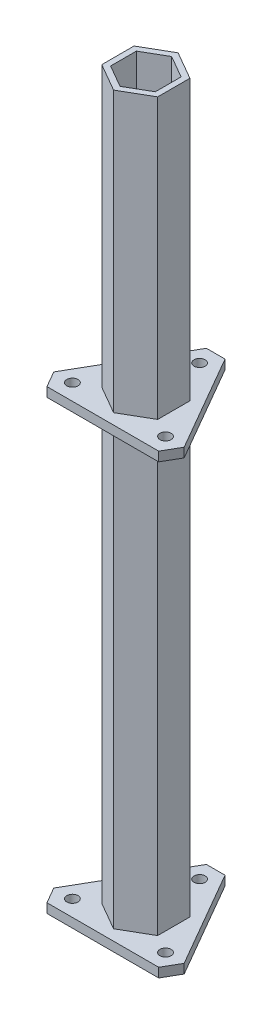
from build123d import *

# Parameters (mm, degrees)
BOSS_EXTRUDE1_DEPTH = 200
BOSS_EXTRUDE2_DEPTH = 5
CUT_EXTRUDE1_DEPTH  = 5
LPATTERN1_COUNT     = 4
LPATTERN1_PITCH     = 120
SKETCH5_R           = 3
CUT_EXTRUDE2_DEPTH  = 399.319386088
CUT_EXTRUDE4_DEPTH  = 10
CUT_EXTRUDE5_DEPTH  = 10


with BuildPart() as part:
    # Sketch1 → Boss-Extrude1 (new, symmetric)
    with BuildSketch(Plane(origin=(0, 0, 0), x_dir=(1, 0, 0), z_dir=(0, 1, 0))):
        Polygon((0, 17.320508076), (-15, 8.660254038), (-15, -8.660254038), (0, -17.320508076), (15, -8.660254038), (15, 8.660254038), align=None)
        Polygon((-12, 6.92820323), (-12, -6.92820323), (0, -13.856406461), (12, -6.92820323), (12, 6.92820323), (0, 13.856406461), align=None, mode=Mode.SUBTRACT)
    extrude(amount=BOSS_EXTRUDE1_DEPTH, both=True)

    # Sketch2 → Boss-Extrude2 (add)
    with BuildSketch(Plane(origin=(0, 170, 0), x_dir=(1, 0, 0), z_dir=(0, 1, 0))):
        Polygon((0, 46.188021535), (-40, -23.094010768), (40, -23.094010768), align=None)
        Polygon((15, 8.660254038), (0, 17.320508076), (-15, 8.660254038), (-15, -8.660254038), (0, -17.320508076), (15, -8.660254038), align=None, mode=Mode.SUBTRACT)
    boss_extrude2 = extrude(amount=-BOSS_EXTRUDE2_DEPTH)

    # Sketch3 → Cut-Extrude1 (cut)
    with BuildSketch(Plane.XZ.offset(-165)):
        Polygon((0, -46.188021535), (5, -37.527767497), (-5, -37.527767497), align=None)
        Polygon((40, 23.094010768), (30, 23.094010768), (35, 14.43375673), align=None)
        Polygon((-40, 23.094010768), (-35, 14.43375673), (-30, 23.094010768), align=None)
    cut_extrude1 = extrude(amount=-CUT_EXTRUDE1_DEPTH, mode=Mode.SUBTRACT)

    # LPattern1: Boss-Extrude2, Cut-Extrude1 ×4
    with Locations(*[(0, -i * LPATTERN1_PITCH, 0) for i in range(1, LPATTERN1_COUNT)]):
        add(boss_extrude2)
        add(cut_extrude1, mode=Mode.SUBTRACT)

    # Sketch5 → Cut-Extrude2 (cut, through all)
    with BuildSketch(Plane.XZ.offset(195)):
        with Locations(Location((-25, 14.43375673, 0), (0, 0, 270))):
            Circle(SKETCH5_R)
        with Locations(Location((25, 14.43375673, 0), (0, 0, 270))):
            Circle(SKETCH5_R)
        with Locations(Location((0, -28.867513459, 0), (0, 0, 270))):
            Circle(SKETCH5_R)
    extrude(amount=-CUT_EXTRUDE2_DEPTH, mode=Mode.SUBTRACT)

    # Sketch7 → Cut-Extrude4 (cut)
    with BuildSketch(Plane.XZ.offset(-165)):
        Polygon((30, 23.094010768), (-30, 23.094010768), (-35, 14.43375673), (-5, -37.527767497), (5, -37.527767497), (35, 14.43375673), align=None)
        Polygon((-15, -8.660254038), (-15, 8.660254038), (0, 17.320508076), (15, 8.660254038), (15, -8.660254038), (0, -17.320508076), align=None, mode=Mode.SUBTRACT)
    extrude(amount=-CUT_EXTRUDE4_DEPTH, mode=Mode.SUBTRACT)

    # Sketch8 → Cut-Extrude5 (cut)
    with BuildSketch(Plane.XZ.offset(75)):
        Polygon((-35, 14.43375673), (-5, -37.527767497), (5, -37.527767497), (35, 14.43375673), (30, 23.094010768), (-30, 23.094010768), align=None)
        Polygon((0, 17.320508076), (15, 8.660254038), (15, -8.660254038), (0, -17.320508076), (-15, -8.660254038), (-15, 8.660254038), align=None, mode=Mode.SUBTRACT)
    extrude(amount=-CUT_EXTRUDE5_DEPTH, mode=Mode.SUBTRACT)


solid = part.part
